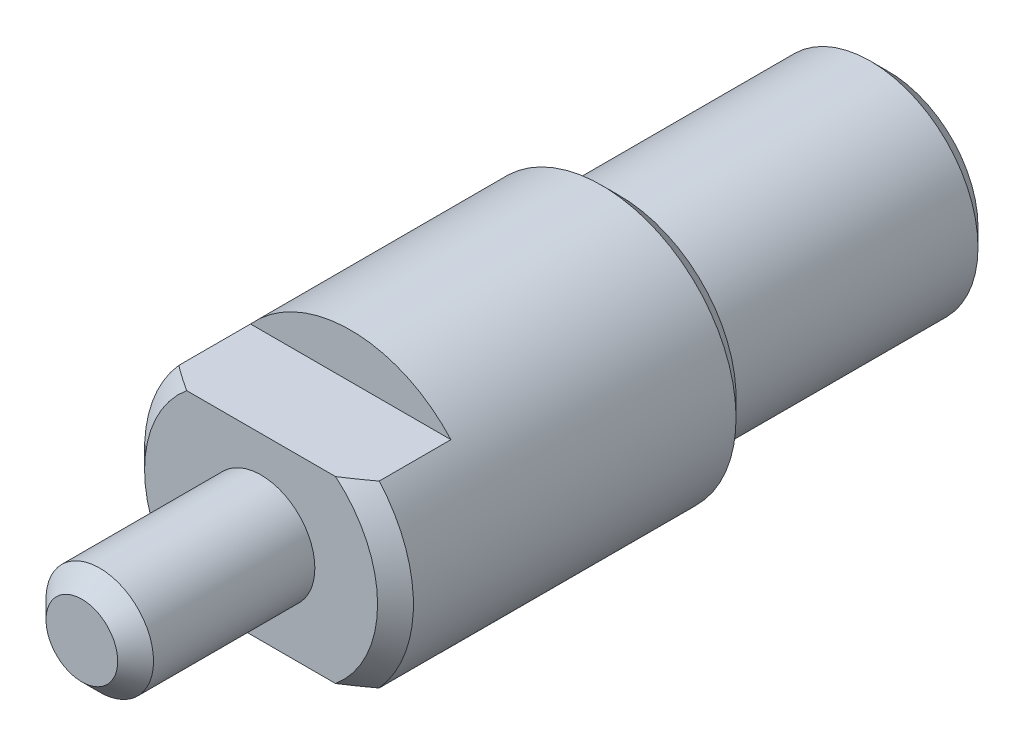
from build123d import *

# Parameters (mm, degrees)
EXTRUDE_1_DEPTH      = 30
EXTRUDE_1_DEPTH_BACK = 15
SKETCH_1_R           = 7.5
SKETCH_2_R           = 7.5
SKETCH_2_R_2         = 3
CUT_EXTRUDE_1_DEPTH  = 10
CHAMFER_1_SIZE       = 1
SKETCH_3_R           = 7.5
SKETCH_3_R_2         = 6
CUT_EXTRUDE_2_DEPTH  = 15
CHAMFER_2_SIZE       = 1
CHAMFER_3_SIZE       = 1
CHAMFER_4_SIZE       = 1
SKETCH_4_W           = 26.213765936
SKETCH_4_H           = 7.269713565
SKETCH_4_W_2         = 30.615700216
SKETCH_4_H_2         = 9.339731857
CUT_EXTRUDE_3_DEPTH  = 5


with BuildPart() as part:
    # 草图1 → 凸台-拉伸1 (new, two sides: drawn at the far end of the back side and taken through both)
    with BuildSketch(Plane.XY.offset(-EXTRUDE_1_DEPTH_BACK)):
        Circle(SKETCH_1_R)
    extrude(amount=EXTRUDE_1_DEPTH + EXTRUDE_1_DEPTH_BACK)

    # 草图2 → 切除-拉伸1 (cut)
    with BuildSketch(Plane.XY.offset(30)):
        Circle(SKETCH_2_R)
        Circle(SKETCH_2_R_2, mode=Mode.SUBTRACT)
    extrude(amount=-CUT_EXTRUDE_1_DEPTH, mode=Mode.SUBTRACT)

    # 倒角1
    chamfer_1_edges = [part.edges().sort_by_distance(p)[0] for p in [
        (-3, 0, 30),
    ]]
    chamfer(chamfer_1_edges, length=CHAMFER_1_SIZE)

    # 草图3 → 切除-拉伸2 (cut)
    with BuildSketch(Plane(origin=(0, 0, -15), x_dir=(-1, 0, 0), z_dir=(0, 0, -1))):
        with Locations(Location((0, 0, 0), (0, 0, 180))):
            Circle(SKETCH_3_R)
        Circle(SKETCH_3_R_2, mode=Mode.SUBTRACT)
    extrude(amount=-CUT_EXTRUDE_2_DEPTH, mode=Mode.SUBTRACT)

    # 倒角2
    chamfer_2_edges = [part.edges().sort_by_distance(p)[0] for p in [
        (6, 0, -15),
    ]]
    chamfer(chamfer_2_edges, length=CHAMFER_2_SIZE)

    # 倒角3
    chamfer_3_edges = [part.edges().sort_by_distance(p)[0] for p in [
        (-7.5, 0, 0),
    ]]
    chamfer(chamfer_3_edges, length=CHAMFER_3_SIZE)

    # 倒角4
    chamfer_4_edges = [part.edges().sort_by_distance(p)[0] for p in [
        (-7.5, 0, 20),
    ]]
    chamfer(chamfer_4_edges, length=CHAMFER_4_SIZE)

    # 草图4 → 切除-拉伸3 (cut)
    with BuildSketch(Plane.XY.offset(20)):
        with Locations((-1.405852491, -8.634856782)):
            Rectangle(SKETCH_4_W, SKETCH_4_H)
        with Locations((-0.14462413, 9.669865929)):
            Rectangle(SKETCH_4_W_2, SKETCH_4_H_2)
    extrude(amount=-CUT_EXTRUDE_3_DEPTH, mode=Mode.SUBTRACT)


solid = part.part
